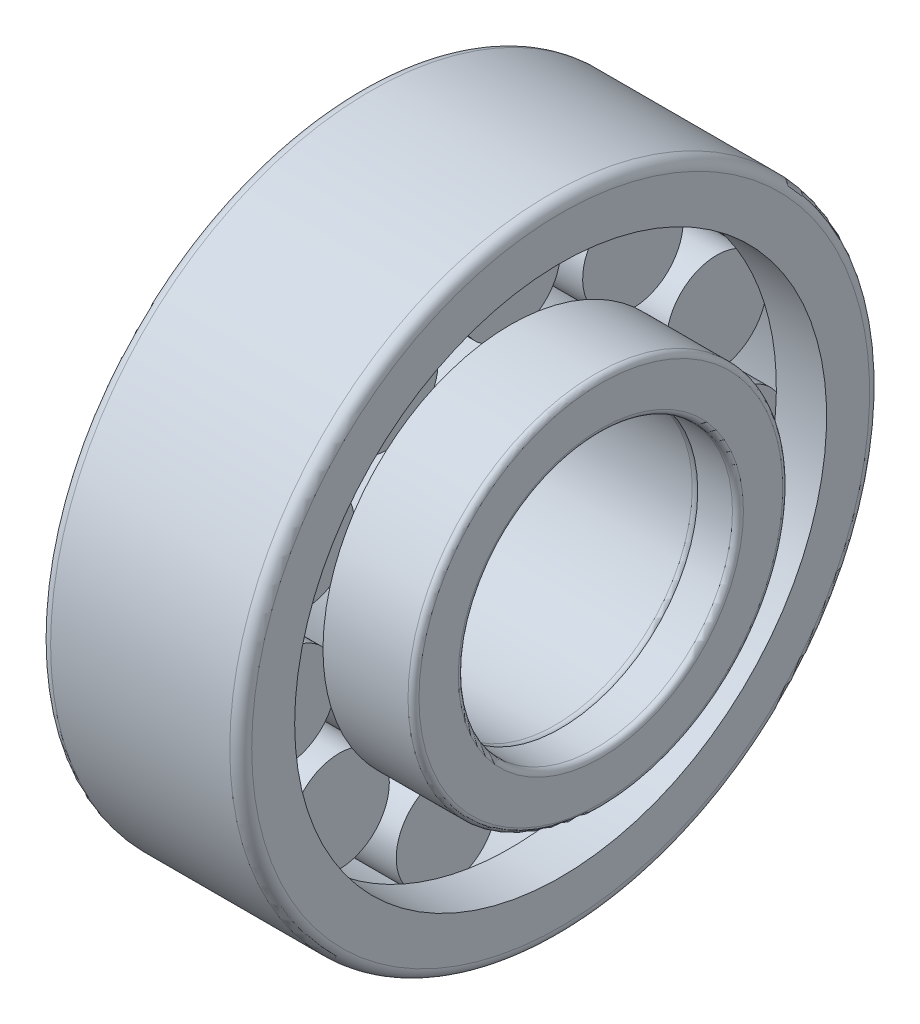
from build123d import *

# Parameters (mm, degrees)
SKETCH_3_W               = 5.5
SKETCH_3_H               = 2.7501
PATTERN_CIRCULAR_1_COUNT = 11


with BuildPart() as part:
    # 草图2 → Revolve 794 (revolve)
    with BuildSketch(Plane.XY, mode=Mode.PRIVATE) as revolve_794_sk:
        with BuildLine():
            Line((2.75, 9.65), (8.25, 9.65))
            Line((8.25, 9.65), (11, 8.913139721))
            Line((11, 8.913139721), (11, 7.8))
            ThreePointArc((11, 7.8), (10.912132034, 7.587867966), (10.7, 7.5))
            Line((10.7, 7.5), (0.3, 7.5))
            ThreePointArc((0.3, 7.5), (0.087867966, 7.587867966), (0, 7.8))
            Line((0, 7.8), (0, 10.25))
            Line((0, 10.25), (2.75, 10.25))
            Line((2.75, 10.25), (2.75, 9.65))
        make_face()
    revolve(revolve_794_sk.sketch.rotate(Axis((-10.080094127, 0, 0), (1, 0, 0)), 90), axis=Axis((-10.080094127, 0, 0), (1, 0, 0)))

    # 草图3 → 凸台-旋转1 (revolve)
    with BuildSketch(Plane.XY):
        with Locations((5.5, 11.02495)):
            Rectangle(SKETCH_3_W, SKETCH_3_H)
    revolve_1 = revolve(axis=Axis((-1.603948851, 12.4, 0), (1, 0, 0)))

    # 草图4 → 凸台-旋转2 (revolve)
    with BuildSketch(Plane.XY, mode=Mode.PRIVATE) as revolve_2_sk:
        with BuildLine():
            Line((8.25, 14.55), (11, 14.55))
            Line((11, 14.55), (11, 16.9))
            ThreePointArc((11, 16.9), (10.824264069, 17.324264069), (10.4, 17.5))
            Line((10.4, 17.5), (0.6, 17.5))
            ThreePointArc((0.6, 17.5), (0.175735931, 17.324264069), (0, 16.9))
            Line((0, 16.9), (0, 14.55))
            Line((0, 14.55), (2.75, 14.55))
            Line((2.75, 14.55), (2.75, 15.15))
            Line((2.75, 15.15), (8.25, 15.15))
            Line((8.25, 15.15), (8.25, 14.55))
        make_face()
    revolve(revolve_2_sk.sketch.rotate(Axis((0, 0, 0), (1, 0, 0)), 90), axis=Axis((0, 0, 0), (1, 0, 0)))

    # 草图5 → 凸台-旋转3 (revolve)
    with BuildSketch(Plane.XY, mode=Mode.PRIVATE) as revolve_3_sk:
        with BuildLine():
            Line((11, 8.913117543), (11, 7.5))
            Line((11, 7.5), (12.9, 7.5))
            ThreePointArc((12.9, 7.5), (13.112132034, 7.587867966), (13.2, 7.8))
            Line((13.2, 7.8), (13.2, 9.95))
            ThreePointArc((13.2, 9.95), (13.112132034, 10.162132034), (12.9, 10.25))
            Line((12.9, 10.25), (8.25, 10.25))
            Line((8.25, 10.25), (8.25, 9.649977822))
            Line((8.25, 9.649977822), (11, 8.913117543))
        make_face()
    revolve(revolve_3_sk.sketch.rotate(Axis((0, 0, 0), (1, 0, 0)), 90), axis=Axis((0, 0, 0), (1, 0, 0)))

    # 阵列(圆周)1: 凸台-旋转1 ×11 about axis
    pattern_circular_1_axis = Axis((0, 0, 0), (1, 0, 0))
    for i in range(1, PATTERN_CIRCULAR_1_COUNT):
        add(revolve_1.rotate(pattern_circular_1_axis, i * 360 / PATTERN_CIRCULAR_1_COUNT))


solid = part.part
